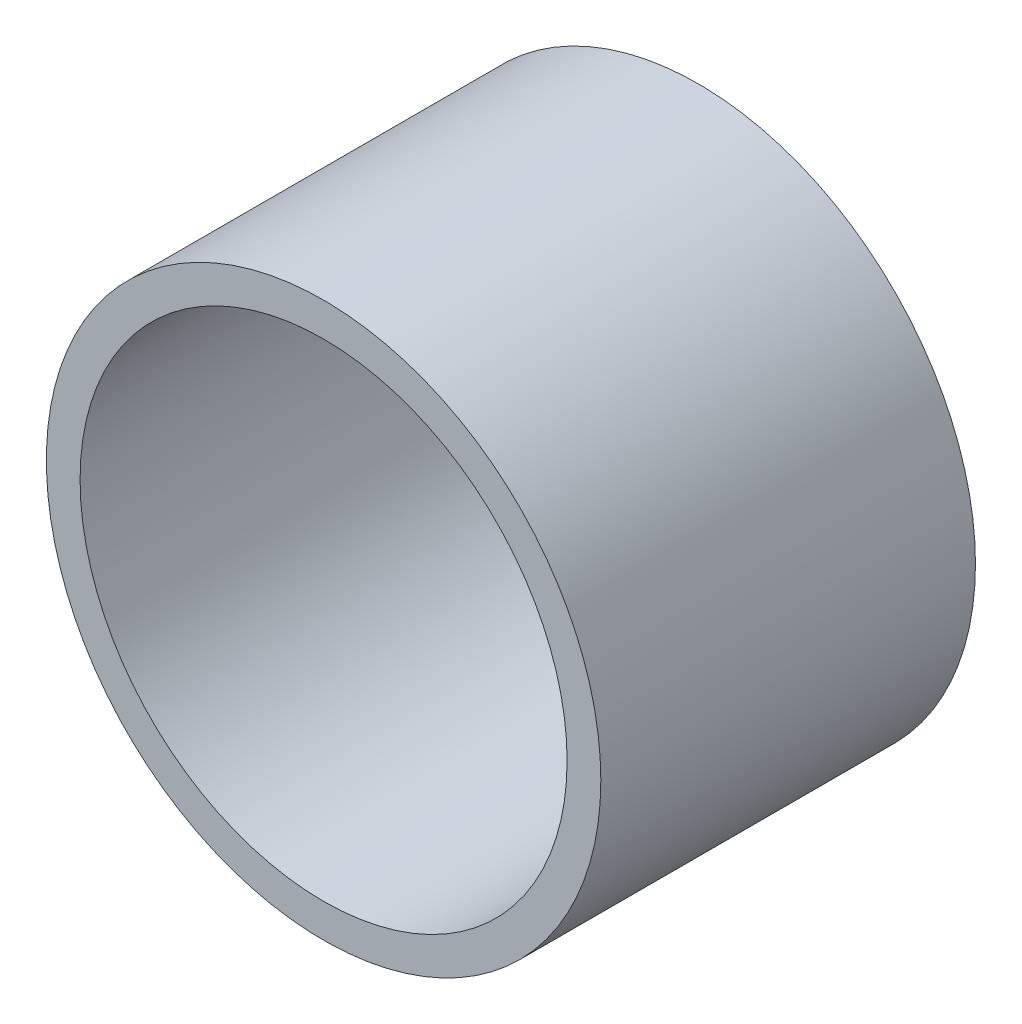
from build123d import *

# Parameters (mm, degrees)
SKETCH_1_R      = 7.4
SKETCH_1_R_2    = 6.5
EXTRUDE_1_DEPTH = 10


with BuildPart() as part:
    # 草图1 → 凸台-拉伸1 (new body)
    with BuildSketch(Plane.XY):
        Circle(SKETCH_1_R)
        Circle(SKETCH_1_R_2, mode=Mode.SUBTRACT)
    extrude(amount=EXTRUDE_1_DEPTH)


solid = part.part
